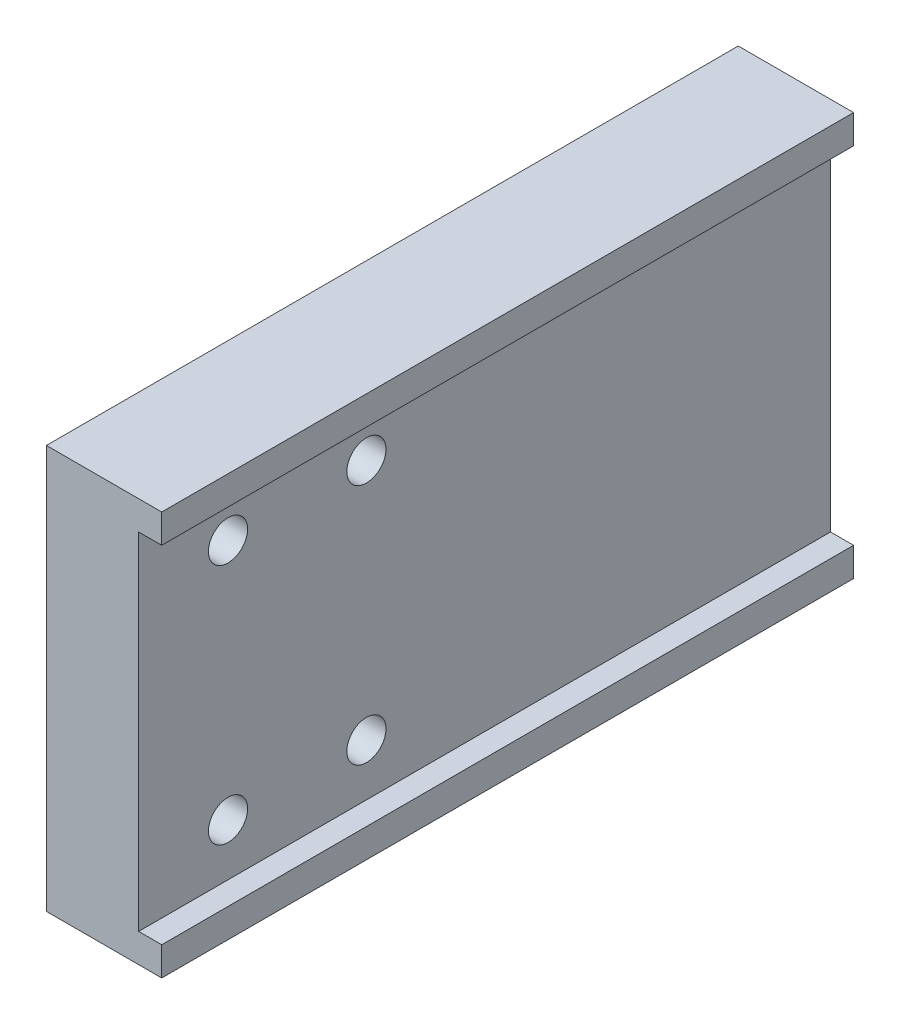
from build123d import *

# Parameters (mm, degrees)
SKETCH1_W                                            = 60
SKETCH1_H                                            = 35
BOSS_EXTRUDE1_DEPTH                                  = 10
SKETCH2_W                                            = 60
SKETCH2_H                                            = 30
CUT_EXTRUDE1_DEPTH                                   = 2
CBORE_FOR_M3_HEXAGON_SOCKET_HEAD_CAP_SCR_D           = 3.4
CBORE_FOR_M3_HEXAGON_SOCKET_HEAD_CAP_SCR_CBORE_D     = 6
CBORE_FOR_M3_HEXAGON_SOCKET_HEAD_CAP_SCR_CBORE_DEPTH = 3.4
M4_TAPPED_HOLE1_D                                    = 3.3
M4_TAPPED_HOLE1_DEPTH                                = 10.1
M4_TAPPED_HOLE1_TIP                                  = 0.991420021


with BuildPart() as part:
    # Sketch1 → Boss-Extrude1 (new body)
    with BuildSketch(Plane(origin=(0, 0, 0), x_dir=(0, 0, -1), z_dir=(1, 0, 0))):
        Rectangle(SKETCH1_W, SKETCH1_H)
    extrude(amount=BOSS_EXTRUDE1_DEPTH)

    # Sketch2 → Cut-Extrude1 (cut)
    with BuildSketch(Plane(origin=(10, 0, 0), x_dir=(0, 0, -1), z_dir=(1, 0, 0))):
        Rectangle(SKETCH2_W, SKETCH2_H)
    extrude(amount=-CUT_EXTRUDE1_DEPTH, mode=Mode.SUBTRACT)

    # CBORE for M3 Hexagon socket head cap screws1 (through all)
    with Locations(Plane.ZY):
        with Locations((22.25, 10.5), (10.25, 10.5), (10.25, -10.5), (22.25, -10.5)):
            CounterBoreHole(CBORE_FOR_M3_HEXAGON_SOCKET_HEAD_CAP_SCR_D / 2, CBORE_FOR_M3_HEXAGON_SOCKET_HEAD_CAP_SCR_CBORE_D / 2, CBORE_FOR_M3_HEXAGON_SOCKET_HEAD_CAP_SCR_CBORE_DEPTH)

    # M4 Tapped Hole1
    with Locations(Plane(origin=(0, 0, -30), x_dir=(-1, 0, 0), z_dir=(0, 0, -1))):
        with Locations((-4, -10), (-4, 10)):
            Hole(M4_TAPPED_HOLE1_D / 2, depth=M4_TAPPED_HOLE1_DEPTH)
            with Locations((0, 0, -(M4_TAPPED_HOLE1_DEPTH + M4_TAPPED_HOLE1_TIP / 2))):  # 118° drill point
                Cone(0, M4_TAPPED_HOLE1_D / 2, M4_TAPPED_HOLE1_TIP, mode=Mode.SUBTRACT)


solid = part.part
